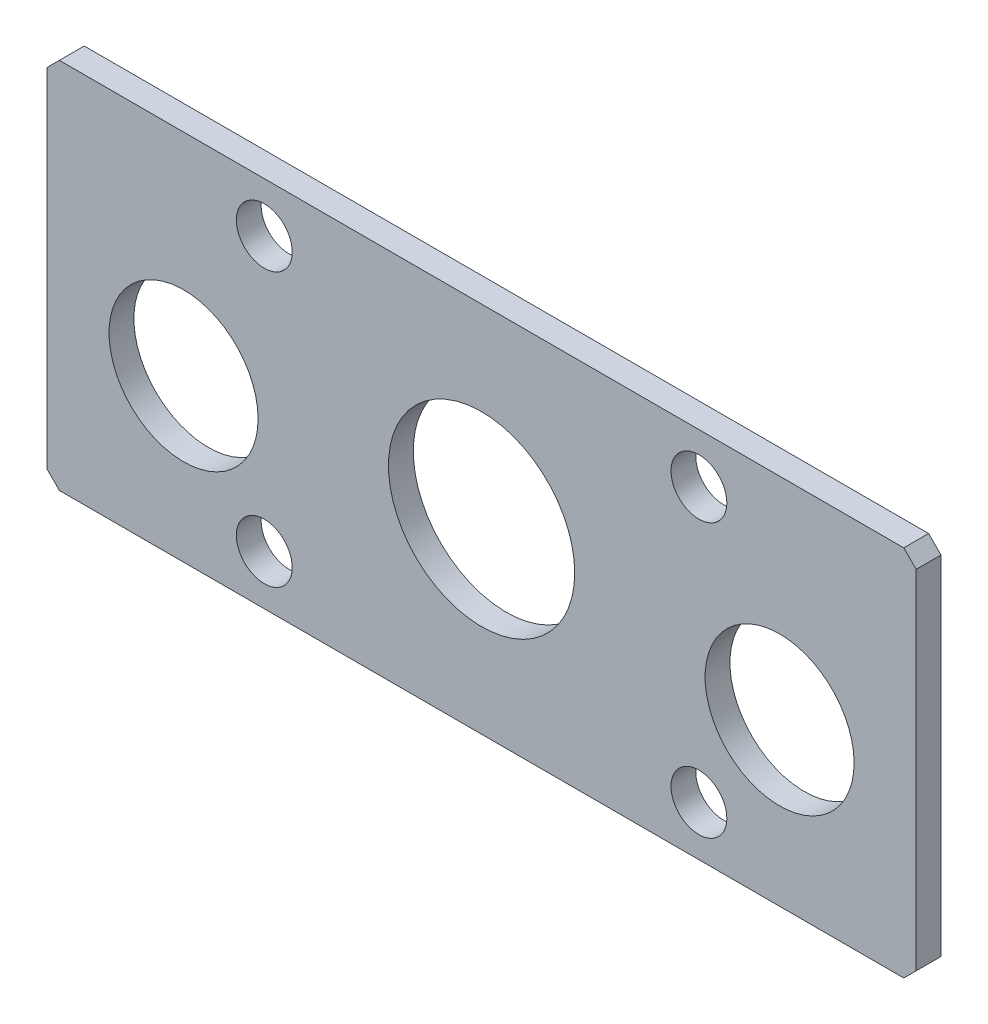
SolidWorks part; units mm, degrees
material "SUS304"
ref_plane "Front Plane" through (0, 0, 0) normal (0, 0, 1) x (1, 0, 0)
ref_plane "Top Plane" through (0, 0, 0) normal (0, 1, 0) x (1, 0, 0)
ref_plane "Right Plane" through (0, 0, 0) normal (1, 0, 0) x (0, 0, -1)
sketch "Sketch1" plane through (0, 0, 0) normal (0, 0, 1) x (1, 0, 0)
  line L1 (35, 30) -> (-35, 30)
  line L2 (35, 30) -> (35, 0)
  line L3 (35, 0) -> (-35, 0)
  line L4 (-35, 30) -> (-35, 0)
  line L5 (0, 15) -> (0, 0) construction
  circle A0 centre (-24, 13) radius 6
  circle A1 centre (24, 13) radius 6
  circle A2 centre (0, 15) radius 7.5
  dimension "D3" = 12
  dimension "D4" = 12
  dimension "D5" = 15
  dimension "D7" = 17
  dimension "D1" = 70
  dimension "D2" = 30
  dimension "D6" = 48
  dimension "D8" = 15
extrude "Boss-Extrude1" add sketch "Sketch1" along normal blind 2
hole_wizard "Ø4.5 (4.5) Diameter Hole1" positions "Sketch3" profile "Sketch2" hole size "Ø4.5" standard "ISO" end condition through all
sketch "Sketch3" plane through (0, 0, 2) normal (0, 0, 1) x (1, 0, 0)
  line L0 (-17.5, 26) -> (17.5, 26) construction
  line L1 (-17.5, 4) -> (17.5, 4) construction
  line L3 (0, 15) -> (0, 26) construction
  line L4 (0, 15) -> (13.1631, 15) construction
  point P0 (-17.5, 26)
  point P3 (17.5, 26)
  point P18 (-17.5, 4)
  point P20 (17.5, 4)
  dimension "D1" = 35
  dimension "D4" = 22
sketch "Sketch2" plane through (-17.5, 26, 2) normal (1, 0, 0) x (0, -1, 0)
  line L0 (0, 0) -> (0, 2)
  line L1 (0, 2) -> (2.25, 2)
  line L2 (2.25, 2) -> (2.25, 0)
  line L5 (2.25, 0) -> (0, 0)
  line L11 (0, -6.35) -> (0, 107.95) construction
  dimension "通孔孔直径" = 4.5
  dimension "通孔孔深度" = 2
chamfer "Chamfer1" distance 1 angle 45 4 edges at (-35, 0, 1) (-35, 30, 1) (35, 30, 1) (35, 0, 1)
